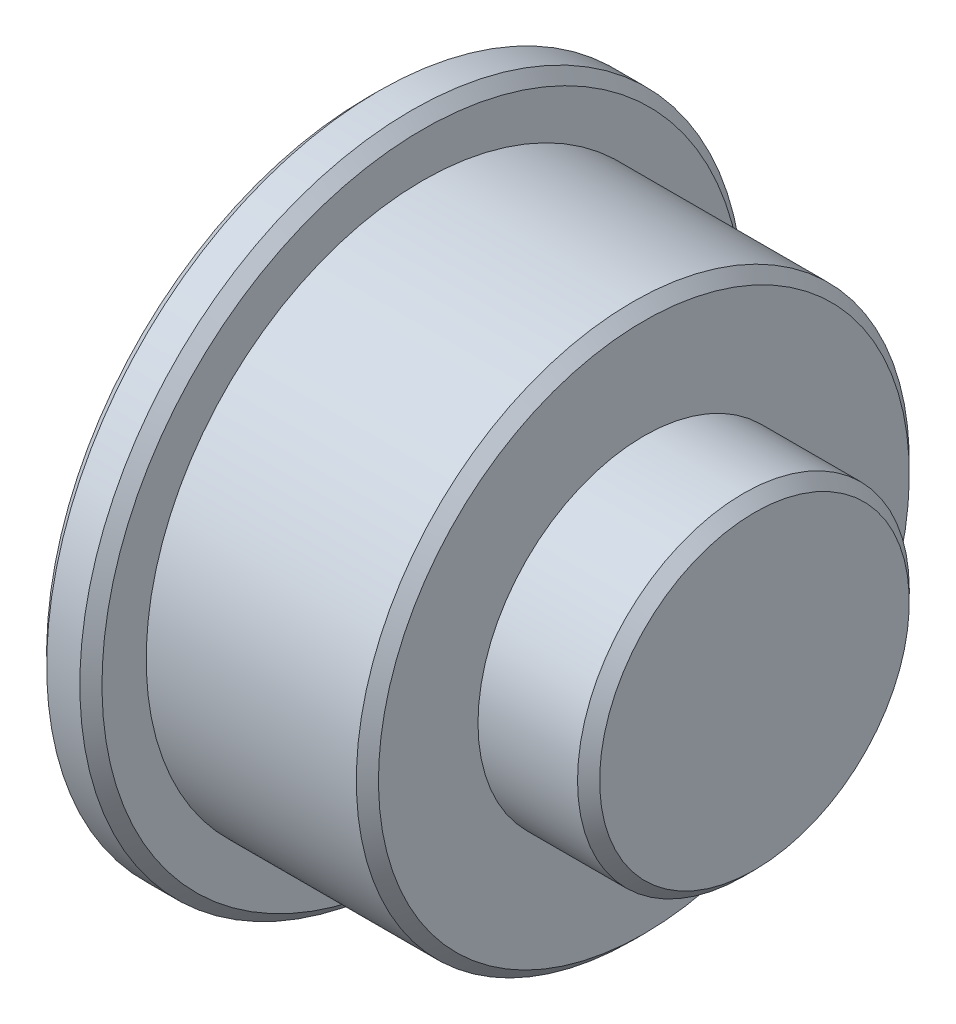
from build123d import *

# Parameters (mm, degrees)
CHAMFER1_SIZE = 1


with BuildPart() as part:
    # Sketch1 → Revolve1 (revolve)
    with BuildSketch(Plane.XY, mode=Mode.PRIVATE) as revolve1_sk:
        Polygon((30, -15), (20, -15), (20, -25), (0, -25), (0, -30), (-5, -30), (-5, 0), (30, 0), align=None)
    revolve(revolve1_sk.sketch.rotate(Axis((30, 0, 0), (-1, 0, 0)), 180), axis=Axis((30, 0, 0), (-1, 0, 0)))

    # Chamfer1
    chamfer1_edges = [part.edges().sort_by_distance(p)[0] for p in [
        (30, -15, 0),
        (20, -25, 0),
        (0, -30, 0),
        (-5, -30, 0),
    ]]
    chamfer(chamfer1_edges, length=CHAMFER1_SIZE)


solid = part.part
